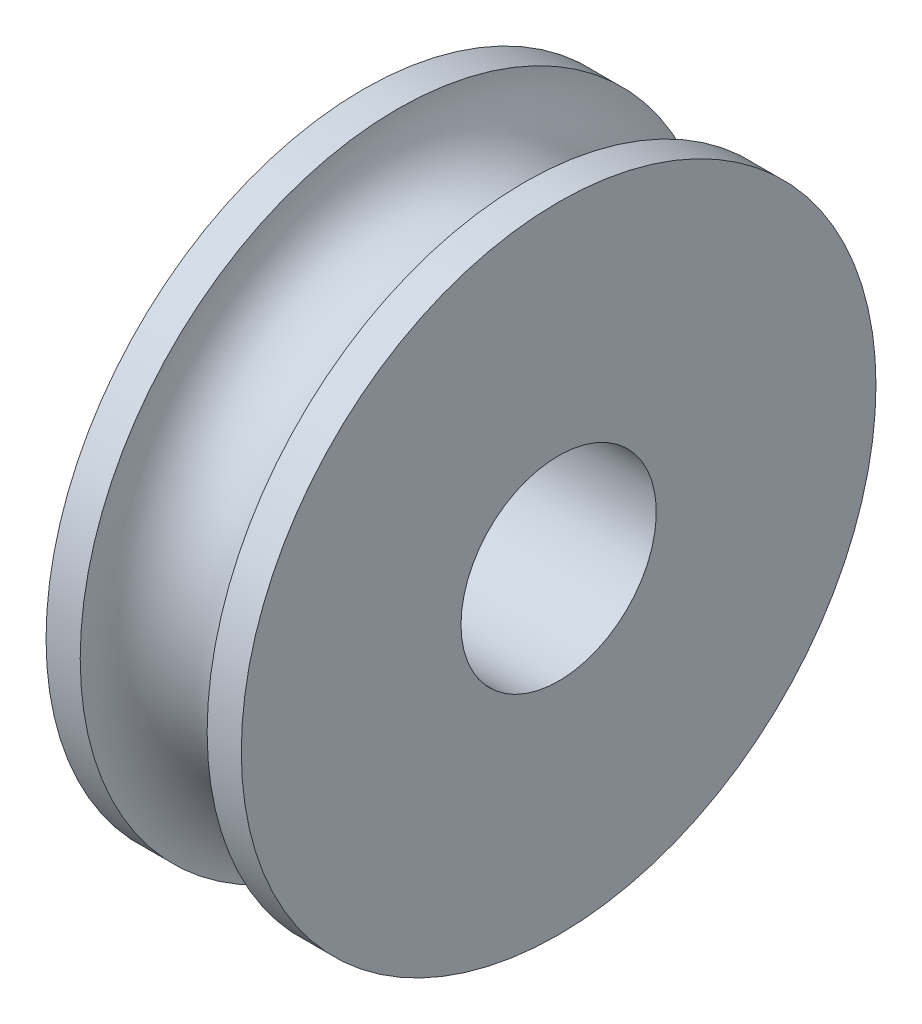
from build123d import *


with BuildPart() as part:
    # Sketch1 → Revolve1 (revolve)
    with BuildSketch(Plane(origin=(0, 0, 0), x_dir=(1, 0, 0), z_dir=(0, 1, 0)), mode=Mode.PRIVATE) as revolve1_sk:
        with BuildLine():
            Line((0, 2), (4, 2))
            Line((4, 2), (4, 6.5))
            Line((4, 6.5), (3.3, 6.5))
            ThreePointArc((3.3, 6.5), (2, 5.2), (0.7, 6.5))
            Line((0.7, 6.5), (0, 6.5))
            Line((0, 6.5), (0, 2))
        make_face()
    revolve(revolve1_sk.sketch.rotate(Axis((0, 0, 0), (1, 0, 0)), 180), axis=Axis((0, 0, 0), (1, 0, 0)))


solid = part.part
